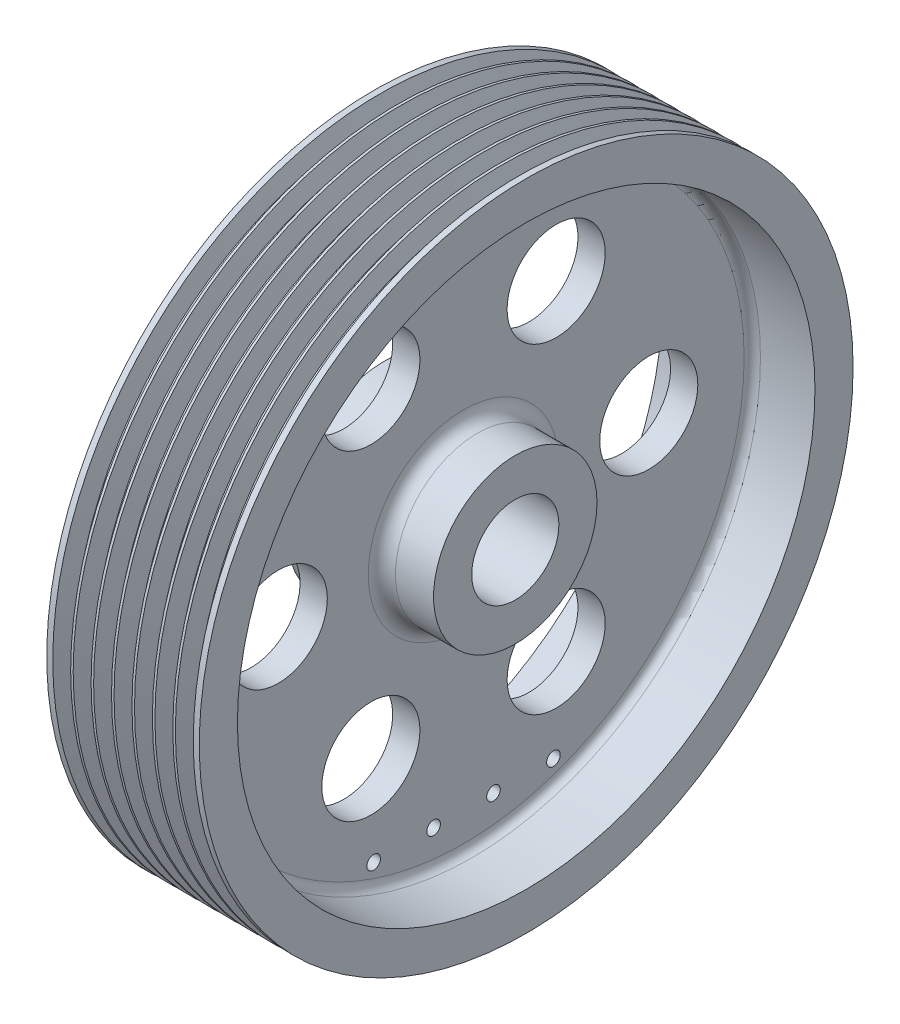
SolidWorks part; units mm, degrees
material "灰铸铁 HT200 "
ref_plane "Front Plane" through (0, 0, 0) normal (0, 0, 1) x (1, 0, 0)
ref_plane "Top Plane" through (0, 0, 0) normal (0, 1, 0) x (1, 0, 0)
ref_plane "Right Plane" through (0, 0, 0) normal (1, 0, 0) x (0, 0, -1)
sketch "Sketch2" plane through (0, 0, 0) normal (0, 0, 1) x (1, 0, 0)
  line L0 (225.6571, 0) -> (0, 0) construction
  line L1 (-20, 600) -> (-20, 530)
  line L2 (260, 600) -> (260, 530)
  line L3 (95, 515) -> (95, 205)
  line L4 (145, 515) -> (145, 175)
  line L5 (0, 180) -> (0, 105)
  line L6 (240, 150) -> (240, 80)
  line L7 (70, 180) -> (0, 180)
  line L8 (170, 150) -> (240, 150)
  line L9 (260, 530) -> (160, 530)
  line L10 (80, 530) -> (-20, 530)
  line L11 (0, 105) -> (70, 105)
  line L12 (70, 105) -> (70, 80)
  line L13 (70, 80) -> (240, 80)
  line L14 (-20, 600) -> (260, 600)
  line L15 (120, 324.3302) -> (120, 85.9832) construction
  arc A0 (145, 175) -> (170, 150) centre (170, 175) ccw
  arc A4 (70, 180) -> (95, 205) centre (70, 205) ccw
  arc A6 (160, 530) -> (145, 515) centre (160, 515) ccw
  arc A7 (95, 515) -> (80, 530) centre (80, 515) ccw
  dimension "D9" = 25
  dimension "D10" = 25
  dimension "D11" = 15
  dimension "D13" = 15
  dimension "D1" = 80
  dimension "D2" = 105
  dimension "D3" = 70
  dimension "D4" = 240
  dimension "D5" = 180
  dimension "D6" = 150
  dimension "D7" = 20
  dimension "D8" = 50
  dimension "D12" = 530
  dimension "D14" = 600
  dimension "D15" = 280
sketch "Sketch3" plane through (538.8474, 0, 0) normal (1, 0, 0) x (0, 0, -1)
  line L0 (0, -1.8755) -> (826.9212, -1.8755) construction
  line L1 (-826.9212, -1.8755) -> (-85, -1.8755) construction
  line L2 (0, 803.1837) -> (0, -867.453) construction
  line L3 (-165.556, 284.8759) -> (-284.8898, 491.5681) construction
  line L4 (-165.556, -288.627) -> (-284.8898, -495.3192) construction
  line L5 (165.556, 284.8759) -> (284.8898, 491.5681) construction
  line L6 (165.556, -288.627) -> (284.8898, -495.3192) construction
  line L7 (-240.2543, 578.1245) -> (242.1135, 578.1245) construction
  line L8 (-60, 620.3139) -> (-60, 535.9351) construction
  line L9 (-180, 621.6856) -> (-180, 534.5633) construction
  line L10 (180, 621.6856) -> (180, 534.5633) construction
  line L11 (60, 620.3139) -> (60, 535.9351) construction
  line L12 (106.8046, 59.7882) -> (151.3767, 85.5219) construction
  line L13 (-103.4525, 57.8528) -> (-149.6234, 84.5096) construction
  line L14 (0, 93.1245) -> (-1, 83.1186)
  line L15 (0, 93.1245) -> (1, 83.1186)
  circle A0 centre (0, 0) radius 450 construction
  circle A1 centre (0, 0) radius 757.5
  circle A2 centre (0, -1.8755) radius 677.5
  circle A3 centre (0, -1.8755) radius 210
  circle A4 centre (0, -1.8755) radius 112.5
  arc A5 (-1, 83.1186) -> (1, 83.1186) centre (0, -1.8755) ccw
  circle A6 centre (-449.9961, -1.8755) radius 60
  circle A7 centre (-224.998, -391.5836) radius 60
  circle A8 centre (224.998, -391.5836) radius 60
  circle A9 centre (449.9961, -1.8755) radius 60
  circle A10 centre (224.998, 387.8325) radius 60
  circle A11 centre (-224.998, 387.8325) radius 60
  circle A12 centre (-180, 578.1245) radius 12.5
  circle A13 centre (-60, 578.1245) radius 12.5
  circle A14 centre (60, 578.1245) radius 12.5
  circle A15 centre (180, 578.1245) radius 12.5
  circle A16 centre (0, -1.8755) radius 145 construction
  circle A17 centre (0, -146.8755) radius 10
  arc A18 (12.9869, -146.2928) -> (0, -159.8755) centre (0, -146.8755) ccw
  arc A19 (131.5625, 59.0861) -> (114.3154, 64.1245) centre (125.5737, 70.6245) ccw
  circle A20 centre (125.5737, 70.6245) radius 10
  arc A21 (-114.3154, 64.1245) -> (-131.5625, 59.0861) centre (-125.5737, 70.6245) ccw
  circle A22 centre (-125.5737, 70.6245) radius 10
revolve "Revolve1" add sketch "Sketch2" angle 360 about L0
sketch "Sketch4" plane through (0, 0, 0) normal (1, 0, 0) x (0, 0, -1)
  line L0 (0, 0) -> (0, 216.8731) construction
  line L1 (0, 0) -> (-210.0698, 363.8516) construction
  circle A0 centre (0, 0) radius 340 construction
  circle A1 centre (-170, 294.4486) radius 90
  dimension "D1" = 680
  dimension "D2" = 180
  dimension "D3" = 30
extrude "Cut-Extrude1" cut sketch "Sketch4" along normal blind 343
pattern_circular "CirPattern1" count 6 over 360 about axis through (0, 0, 0) along (1, 0, 0) of "Cut-Extrude1"
sketch "Sketch5" plane through (0, 0, 0) normal (-1, 0, 0) x (0, 0, 1)
  line L0 (0, 0) -> (66.25, 0) construction
  line L1 (0, 0) -> (66.25, 114.7484) construction
  dimension "D1" = 60
  dimension "D2" = 132.5
hole_wizard "M24 Tapped Hole1" positions "3DSketch1" profile "Sketch6" tap size "M24" standard "GB"
sketch3d "3DSketch1"
  point P0 (0, 114.7484, 66.25)
sketch "Sketch6" plane through (0, 114.7484, 66.25) normal (0, 1, 0) x (0, 0, 1)
  line L0 (0, 0) -> (0, 46.309)
  line L1 (0, 46.309) -> (10.5, 40)
  line L2 (10.5, 40) -> (10.5, 0)
  line L5 (10.5, 0) -> (0, 0)
  line L10 (0, 46.309) -> (-10.5, 40) construction
  line L11 (0, -6.35) -> (0, 107.95) construction
  dimension "螺纹孔钻头直径" = 21
  dimension "螺纹孔钻头深度" = 40
  dimension "导头角度" = 118
cosmetic thread "hole cosmetic thread 1" parameters "D1"=40, "D2"=24
pattern_circular "CirPattern2" count 3 over 360 about axis through (0, 0, 0) along (1, 0, 0) of "M24 Tapped Hole1"
sketch "Sketch8" plane through (0, 0, 0) normal (1, 0, 0) x (0, 0, -1)
  line L0 (0, 0) -> (0, -462) construction
  line L1 (165, -462) -> (-165, -462) construction
  circle A0 centre (-55, -462) radius 12.5
  circle A1 centre (-165, -462) radius 12.5
  circle A2 centre (55, -462) radius 12.5
  circle A3 centre (165, -462) radius 12.5
  point P6 (0, -462)
  dimension "D2" = 25
  dimension "D3" = 110
  dimension "D1" = 462
  dimension "D4" = 55
extrude "Cut-Extrude3" cut sketch "Sketch8" along normal blind 238
sketch "Sketch9" plane through (0, 0, 0) normal (0, 0, 1) x (1, 0, 0)
  line L0 (120, 600) -> (120, 299.5083) construction
  line L2 (260, 600) -> (-20, 600) construction
  line L3 (-8.9268, 600) -> (0.8866, 571.5)
  line L4 (0.8866, 571.5) -> (14.1134, 571.5)
  line L5 (14.1134, 571.5) -> (23.9268, 600)
  line L6 (23.9268, 600) -> (-8.9268, 600)
  line L7 (7.5, 571.5) -> (7.5, 645.9363) construction
  line L8 (-20, 600) -> (-20, -600) construction
  line L9 (-20, 591.5) -> (21, 591.5) construction
  line L10 (-20, 591.5) -> (-20, 600) construction
  line L11 (0, 0) -> (291.0675, 0) construction
  point P12 (-6, 591.5)
  dimension "D1" = 27.5
  dimension "D2" = 38
  dimension "D3" = 28.5
  dimension "D4" = 8.5
  dimension "D5" = 27
revolve "Cut-Revolve1" cut sketch "Sketch9" angle 360 about L11
pattern_linear "LPattern1" count 7 spacing 37.5 along (1, 0, 0) of "Cut-Revolve1"
